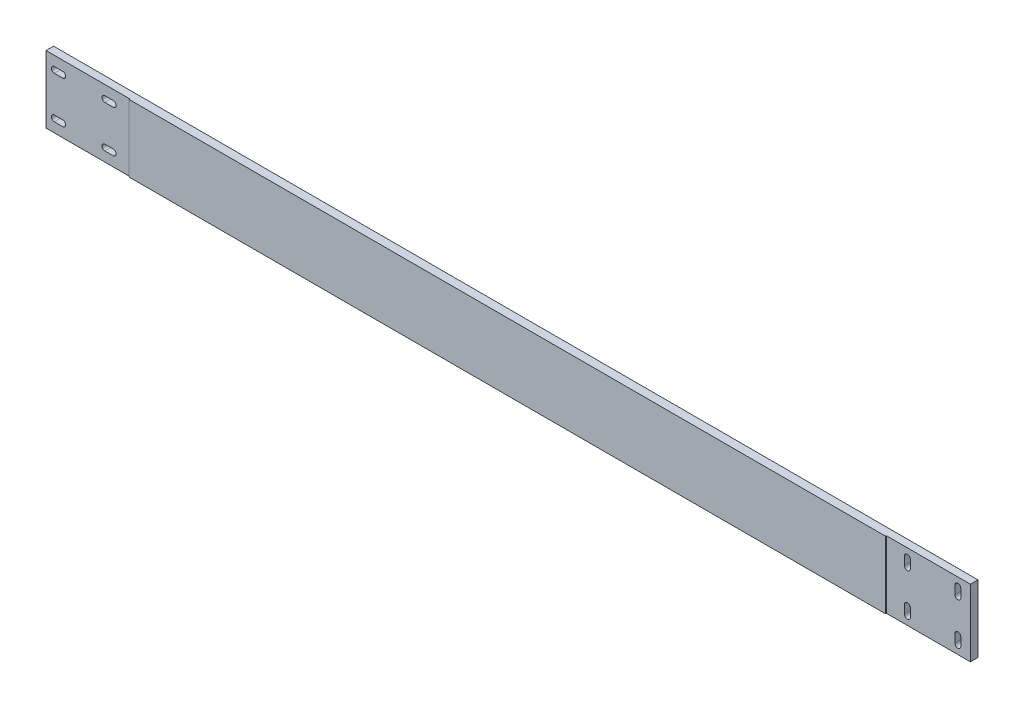
SolidWorks part; units mm, degrees
material "T2"
ref_plane "前视基准面" through (0, 0, 0) normal (0, 0, 1) x (1, 0, 0)
ref_plane "上视基准面" through (0, 0, 0) normal (0, 1, 0) x (1, 0, 0)
ref_plane "右视基准面" through (0, 0, 0) normal (1, 0, 0) x (0, 0, -1)
sketch "草图1" plane through (0, 0, 0) normal (0, 0, 1) x (1, 0, 0)
  line L1 (-550, 40) -> (550, 40)
  line L2 (-550, 40) -> (-550, -40)
  line L3 (-550, -40) -> (550, -40)
  line L4 (550, 40) -> (550, -40)
  line L5 (0, -40) -> (0, 40) construction
  line L6 (-550, 0) -> (550, 0) construction
  point P0 (0, 0)
  dimension "D1" = 80
  dimension "D2" = 1100
extrude "凸台-拉伸1" add sketch "草图1" along normal blind 10
sketch "草图2" plane through (0, 0, 10) normal (0, 0, 1) x (1, 0, 0)
  line L0 (-550, -40) -> (550, -40) construction
  line L1 (-550, 40) -> (-450, 40)
  line L2 (-550, 40) -> (-550, -40)
  line L3 (-550, -40) -> (-450, -40)
  line L4 (-450, 40) -> (-450, -40)
  line L5 (0, 40) -> (0, -40) construction
  line L6 (550, 40) -> (-550, 40) construction
  line L7 (450, 40) -> (450, -40)
  line L8 (550, -40) -> (450, -40)
  line L9 (550, 40) -> (550, -40)
  line L10 (550, 40) -> (450, 40)
  dimension "D1" = 100
extrude "切除-拉伸1" cut sketch "草图2" against normal blind 1
hole_wizard "M6 间隙孔1" positions "草图3" profile "草图4" hole size "M6" standard "GB"
sketch "草图3" plane through (0, 0, 0) normal (0, 0, -1) x (-1, 0, 0)
  line L0 (450, 0) -> (550, 0) construction
  line L1 (450, -40) -> (450, 40) construction
  line L2 (550, 40) -> (550, -40) construction
  line L7 (535, 25) -> (475, 25) construction
  line L8 (535, 25) -> (535, -25) construction
  line L9 (535, -25) -> (475, -25) construction
  line L10 (475, 25) -> (475, -25) construction
  line L11 (505, -25) -> (505, 25) construction
  line L12 (535, 0) -> (475, 0) construction
  line L13 (0, -40) -> (0, 40) construction
  line L14 (550, -40) -> (-550, -40) construction
  line L15 (-550, 40) -> (550, 40) construction
  line L16 (-535, 0) -> (-475, 0) construction
  line L17 (-505, -25) -> (-505, 25) construction
  line L18 (-475, 25) -> (-475, -25) construction
  line L19 (-535, -25) -> (-475, -25) construction
  line L20 (-535, 25) -> (-535, -25) construction
  line L21 (-535, 25) -> (-475, 25) construction
  line L22 (-450, 0) -> (-550, 0) construction
  point P15 (475, -25)
  point P214 (535, 25)
  point P215 (535, -25)
  point P216 (475, 25)
  point P243 (-475, 25)
  point P244 (-475, -25)
  point P245 (-535, -25)
  point P246 (-535, 25)
  dimension "D1" = 60
  dimension "D2" = 50
  dimension "D3" = 25
sketch "草图4" plane through (535, 25, 0) normal (1, 0, 0) x (0, 1, 0)
  line L0 (0, 0) -> (0, 24.353)
  line L1 (0, 24.353) -> (3.5, 22.25)
  line L2 (3.5, 22.25) -> (3.5, 0)
  line L5 (3.5, 0) -> (0, 0)
  line L10 (0, 24.353) -> (-3.5, 22.25) construction
  line L11 (0, -6.35) -> (0, 107.95) construction
  dimension "孔直径" = 7
  dimension "孔深度" = 22.25
  dimension "导头角度" = 118
sketch "草图5" plane through (0, 0, 0) normal (0, 0, -1) x (-1, 0, 0)
  line L0 (470, 25) -> (480, 25) construction
  line L1 (470, 28.5) -> (480, 28.5)
  line L2 (470, 21.5) -> (480, 21.5)
  line L3 (530, 25) -> (540, 25) construction
  line L4 (530, 28.5) -> (540, 28.5)
  line L5 (530, 21.5) -> (540, 21.5)
  line L6 (530, -25) -> (540, -25) construction
  line L7 (530, -21.5) -> (540, -21.5)
  line L8 (530, -28.5) -> (540, -28.5)
  line L9 (470, -25) -> (480, -25) construction
  line L10 (470, -21.5) -> (480, -21.5)
  line L11 (470, -28.5) -> (480, -28.5)
  line L12 (-535, 30) -> (-535, 20) construction
  line L13 (-531.5, 30) -> (-531.5, 20)
  line L14 (-538.5, 30) -> (-538.5, 20)
  line L15 (-475, 30) -> (-475, 20) construction
  line L16 (-471.5, 30) -> (-471.5, 20)
  line L17 (-478.5, 30) -> (-478.5, 20)
  line L18 (-535, -30) -> (-535, -20) construction
  line L19 (-538.5, -30) -> (-538.5, -20)
  line L20 (-531.5, -30) -> (-531.5, -20)
  line L21 (-475, -30) -> (-475, -20) construction
  line L22 (-478.5, -30) -> (-478.5, -20)
  line L23 (-471.5, -30) -> (-471.5, -20)
  arc A0 (470, 28.5) -> (470, 21.5) centre (470, 25) ccw
  arc A1 (480, 21.5) -> (480, 28.5) centre (480, 25) ccw
  arc A2 (530, 28.5) -> (530, 21.5) centre (530, 25) ccw
  arc A3 (540, 21.5) -> (540, 28.5) centre (540, 25) ccw
  arc A4 (530, -21.5) -> (530, -28.5) centre (530, -25) ccw
  arc A5 (540, -28.5) -> (540, -21.5) centre (540, -25) ccw
  arc A6 (470, -21.5) -> (470, -28.5) centre (470, -25) ccw
  arc A7 (480, -28.5) -> (480, -21.5) centre (480, -25) ccw
  arc A8 (-531.5, 30) -> (-538.5, 30) centre (-535, 30) ccw
  arc A9 (-538.5, 20) -> (-531.5, 20) centre (-535, 20) ccw
  arc A10 (-471.5, 30) -> (-478.5, 30) centre (-475, 30) ccw
  arc A11 (-478.5, 20) -> (-471.5, 20) centre (-475, 20) ccw
  arc A12 (-538.5, -30) -> (-531.5, -30) centre (-535, -30) ccw
  arc A13 (-531.5, -20) -> (-538.5, -20) centre (-535, -20) ccw
  arc A14 (-478.5, -30) -> (-471.5, -30) centre (-475, -30) ccw
  arc A15 (-471.5, -20) -> (-478.5, -20) centre (-475, -20) ccw
  point P2 (475, 25)
  point P9 (535, 25)
  point P17 (535, -25)
  point P25 (475, -25)
  point P33 (-535, 25)
  point P41 (-475, 25)
  point P49 (-535, -25)
  point P57 (-475, -25)
  dimension "D1" = 7
  dimension "D2" = 10
extrude "切除-拉伸2" cut sketch "草图5" against normal through all
